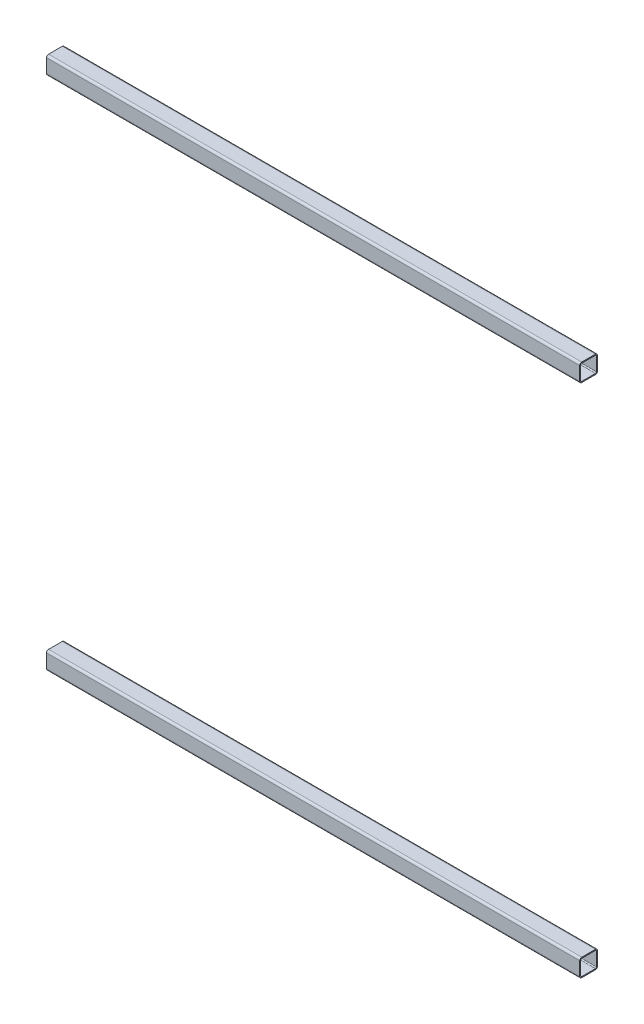
SolidWorks part; units mm, degrees
material "Q235"
ref_plane "Front" through (0, 0, 0) normal (0, 0, 1) x (1, 0, 0)
ref_plane "Top" through (0, 0, 0) normal (0, 1, 0) x (1, 0, 0)
ref_plane "Right" through (0, 0, 0) normal (1, 0, 0) x (0, 0, -1)
sketch "Sketch1" plane through (0, 0, 0) normal (0, 0, 1) x (1, 0, 0)
  line L0 (0, 0) -> (1200, 0)
  line L1 (0, 0) -> (0, 1160)
  line L3 (1200, 1160) -> (1200, 0)
  line L5 (1200, 1160) -> (1200, 0)
  line L6 (0, 1160) -> (1200, 1160)
  dimension "D2" = 1160
  dimension "D3" = 1200
other "Square Tube 40 X 40 X 2.3(1)"
ref_plane "Plane1" through (0, 0, 0) normal (1, 0, 0) x (0, 1, 0)
sketch "Sketch11" plane through (0, 0, 0) normal (1, 0, 0) x (0, 1, 0)
  line L0 (-15.4, -17.7) -> (15.4, -17.7)
  line L1 (-17.7, -15.4) -> (-17.7, 15.4)
  line L2 (15.4, 17.7) -> (-15.4, 17.7)
  line L3 (17.7, 15.4) -> (17.7, -15.4)
  line L4 (-15.4, -20) -> (15.4, -20)
  line L5 (-20, -15.4) -> (-20, 15.4)
  line L6 (15.4, 20) -> (-15.4, 20)
  line L7 (20, 15.4) -> (20, -15.4)
  line L8 (-20, 0) -> (-17.7, 0) construction
  line L9 (-17.7, 0) -> (17.7, 0) construction
  line L10 (17.7, 0) -> (20, 0) construction
  line L12 (0, 20) -> (0, 17.7) construction
  line L13 (0, 17.7) -> (0, -17.7) construction
  line L14 (0, -17.7) -> (0, -20) construction
  arc A0 (20, 15.4) -> (15.4, 20) centre (15.4, 15.4) ccw
  arc A1 (15.4, -20) -> (20, -15.4) centre (15.4, -15.4) ccw
  arc A2 (-20, -15.4) -> (-15.4, -20) centre (-15.4, -15.4) ccw
  arc A3 (-15.4, 20) -> (-20, 15.4) centre (-15.4, 15.4) ccw
  arc A4 (-15.4, 17.7) -> (-17.7, 15.4) centre (-15.4, 15.4) ccw
  arc A5 (17.7, 15.4) -> (15.4, 17.7) centre (15.4, 15.4) ccw
  arc A6 (15.4, -17.7) -> (17.7, -15.4) centre (15.4, -15.4) ccw
  arc A7 (-17.7, -15.4) -> (-15.4, -17.7) centre (-15.4, -15.4) ccw
  point P2 (-20, 20)
  point P33 (-20, -20)
  point P34 (20, -20)
  point P36 (20, 20)
  point P37 (0, 0)
  dimension "D1" = 4.6
  dimension "Thickness" = 2.3
  dimension "V_leg" = 40
  dimension "H_leg" = 40
